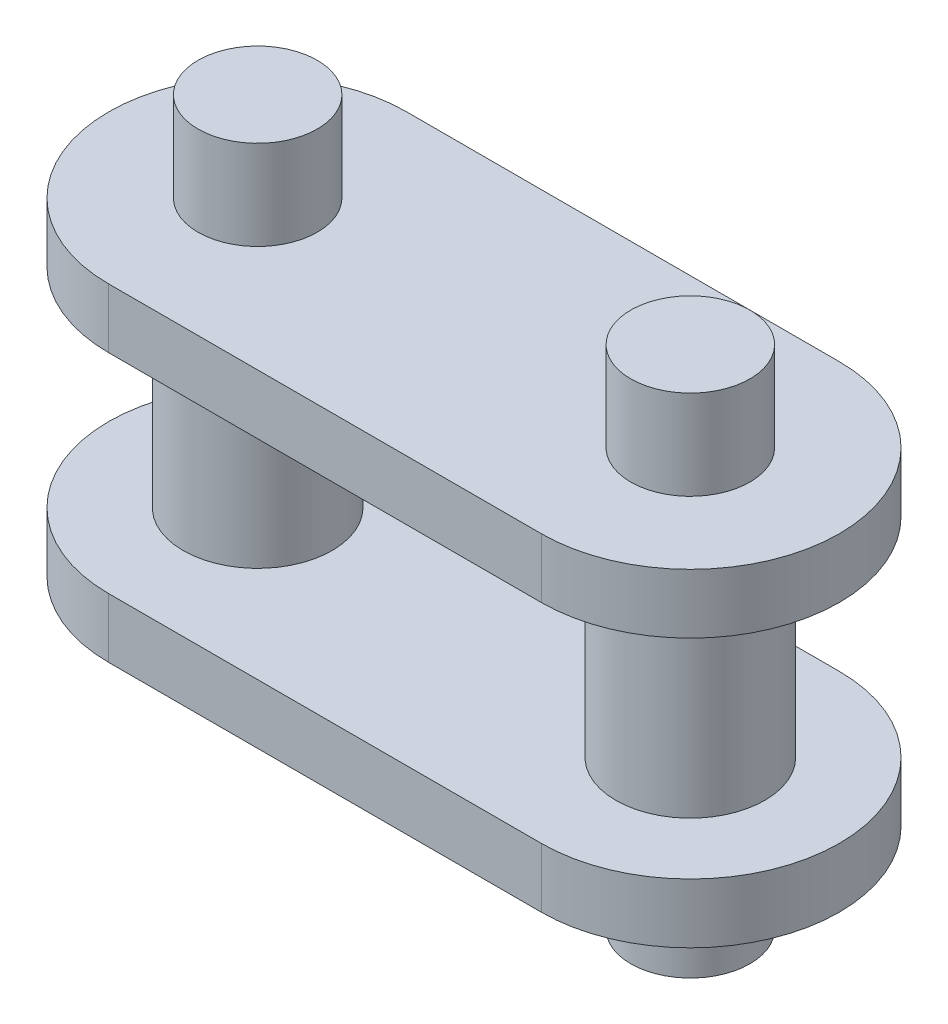
from build123d import *

# Parameters (mm, degrees)
BOSS_EXTRUDE1_DEPTH = 2
SKETCH2_R           = 2.5
BOSS_EXTRUDE2_DEPTH = 7
BOSS_EXTRUDE3_DEPTH = 2
SKETCH4_R           = 2
BOSS_EXTRUDE4_DEPTH = 3
BOSS_EXTRUDE5_START = 3
SKETCH5_R           = 2
BOSS_EXTRUDE5_DEPTH = 3


with BuildPart() as part:
    # Sketch1 → Boss-Extrude1 (new body)
    with BuildSketch(Plane(origin=(0, 0, 0), x_dir=(1, 0, 0), z_dir=(0, 1, 0))):
        with BuildLine():
            Line((0, 5), (14.52, 5))
            ThreePointArc((14.52, 5), (19.52, 0), (14.52, -5))
            Line((14.52, -5), (0, -5))
            ThreePointArc((0, -5), (-5, 0), (0, 5))
        make_face()
    extrude(amount=BOSS_EXTRUDE1_DEPTH)

    # Sketch2 → Boss-Extrude2 (add)
    with BuildSketch(Plane(origin=(0, 2, 0), x_dir=(1, 0, 0), z_dir=(0, 1, 0))):
        with Locations(Location((0, 0, 0), (0, 0, 270))):
            Circle(SKETCH2_R)
        with Locations(Location((14.52, 0, 0), (0, 0, 270))):
            Circle(SKETCH2_R)
    extrude(amount=BOSS_EXTRUDE2_DEPTH)

    # Sketch3 → Boss-Extrude3 (add)
    with BuildSketch(Plane(origin=(0, 9, 0), x_dir=(1, 0, 0), z_dir=(0, 1, 0))):
        with BuildLine():
            Line((0, 5), (14.52, 5))
            ThreePointArc((14.52, 5), (19.52, 0), (14.52, -5))
            Line((14.52, -5), (0, -5))
            ThreePointArc((0, -5), (-5, 0), (0, 5))
        make_face()
    extrude(amount=BOSS_EXTRUDE3_DEPTH)

    # Sketch4 → Boss-Extrude4 (add)
    with BuildSketch(Plane(origin=(0, 11, 0), x_dir=(1, 0, 0), z_dir=(0, 1, 0))):
        with Locations(Location((0, 0, 0), (0, 0, 270))):
            Circle(SKETCH4_R)
        with Locations(Location((14.52, 0, 0), (0, 0, 270))):
            Circle(SKETCH4_R)
    extrude(amount=BOSS_EXTRUDE4_DEPTH)

    # Sketch5 → Boss-Extrude5 (add)
    with BuildSketch(Plane.XZ.offset(BOSS_EXTRUDE5_START)):
        with Locations(Location((0, 0, 0), (0, 0, 90))):
            Circle(SKETCH5_R)
        with Locations(Location((14.52, 0, 0), (0, 0, 90))):
            Circle(SKETCH5_R)
    extrude(amount=-BOSS_EXTRUDE5_DEPTH)


solid = part.part
